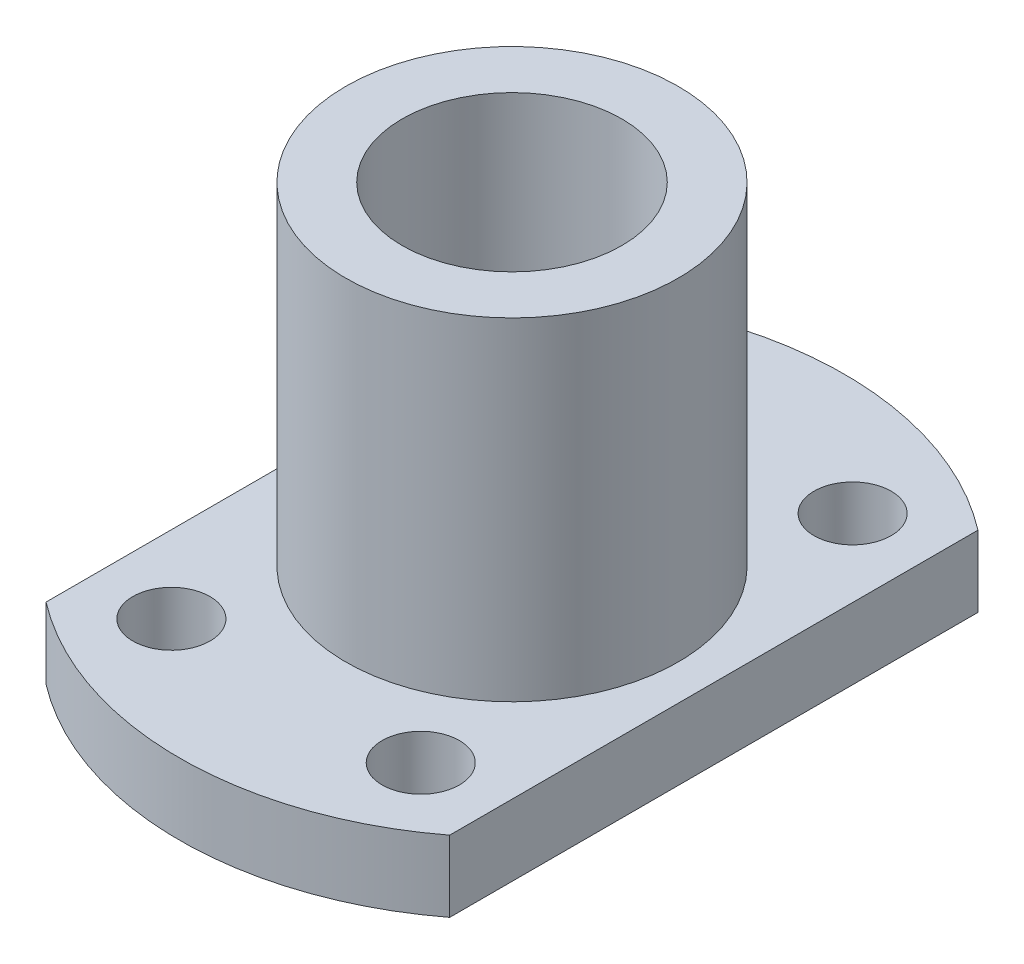
from build123d import *

# Parameters (mm, degrees)
SKETCH2_OUTSIDE_W              = 75.238
SKETCH2_OUTSIDE_H              = 75.238
SKETCH2_OUTSIDE_W_2            = 34
SKETCH2_OUTSIDE_H_2            = 60
CUT_EXTRUDE1_DEPTH             = 10
F_6_5_6_5_DIAMETER_HOLE1_D     = 6.5
F_6_5_6_5_DIAMETER_HOLE1_DEPTH = 20
F_6_5_6_5_DIAMETER_HOLE1_TIP   = 1.952797012
M20X1_5_TAPPED_HOLE1_D         = 18.5
M20X1_5_TAPPED_HOLE1_DEPTH     = 44.5
M20X1_5_TAPPED_HOLE1_TIP       = 5.557960726


with BuildPart() as part:
    # Sketch1 → Revolve1 (revolve)
    with BuildSketch(Plane.XY, mode=Mode.PRIVATE) as revolve1_sk:
        Polygon((0, 0), (28, 0), (28, 6), (14, 6), (14, 34), (0, 34), align=None)
    revolve(revolve1_sk.sketch.rotate(Axis((0, 34, 0), (0, -1, 0)), 180), axis=Axis((0, 34, 0), (0, -1, 0)))

    # Sketch2 outside → Cut-Extrude1 (cut)
    with BuildSketch(Plane.XZ):
        Rectangle(SKETCH2_OUTSIDE_W, SKETCH2_OUTSIDE_H)
        Rectangle(SKETCH2_OUTSIDE_W_2, SKETCH2_OUTSIDE_H_2, mode=Mode.SUBTRACT)
    extrude(amount=-CUT_EXTRUDE1_DEPTH, mode=Mode.SUBTRACT)

    # Ø6.5 (6.5) Diameter Hole1
    with Locations(Plane.XZ):
        with Locations((-10.5, 18.186533479), (10.5, 18.186533479), (-10.5, -18.186533479), (10.5, -18.186533479)):
            Hole(F_6_5_6_5_DIAMETER_HOLE1_D / 2, depth=F_6_5_6_5_DIAMETER_HOLE1_DEPTH)
            with Locations((0, 0, -(F_6_5_6_5_DIAMETER_HOLE1_DEPTH + F_6_5_6_5_DIAMETER_HOLE1_TIP / 2))):  # 118° drill point
                Cone(0, F_6_5_6_5_DIAMETER_HOLE1_D / 2, F_6_5_6_5_DIAMETER_HOLE1_TIP, mode=Mode.SUBTRACT)

    # M20x1.5 Tapped Hole1
    with Locations(Plane.XZ):
        with Locations((0, 0)):
            Hole(M20X1_5_TAPPED_HOLE1_D / 2, depth=M20X1_5_TAPPED_HOLE1_DEPTH)
            with Locations((0, 0, -(M20X1_5_TAPPED_HOLE1_DEPTH + M20X1_5_TAPPED_HOLE1_TIP / 2))):  # 118° drill point
                Cone(0, M20X1_5_TAPPED_HOLE1_D / 2, M20X1_5_TAPPED_HOLE1_TIP, mode=Mode.SUBTRACT)


solid = part.part
